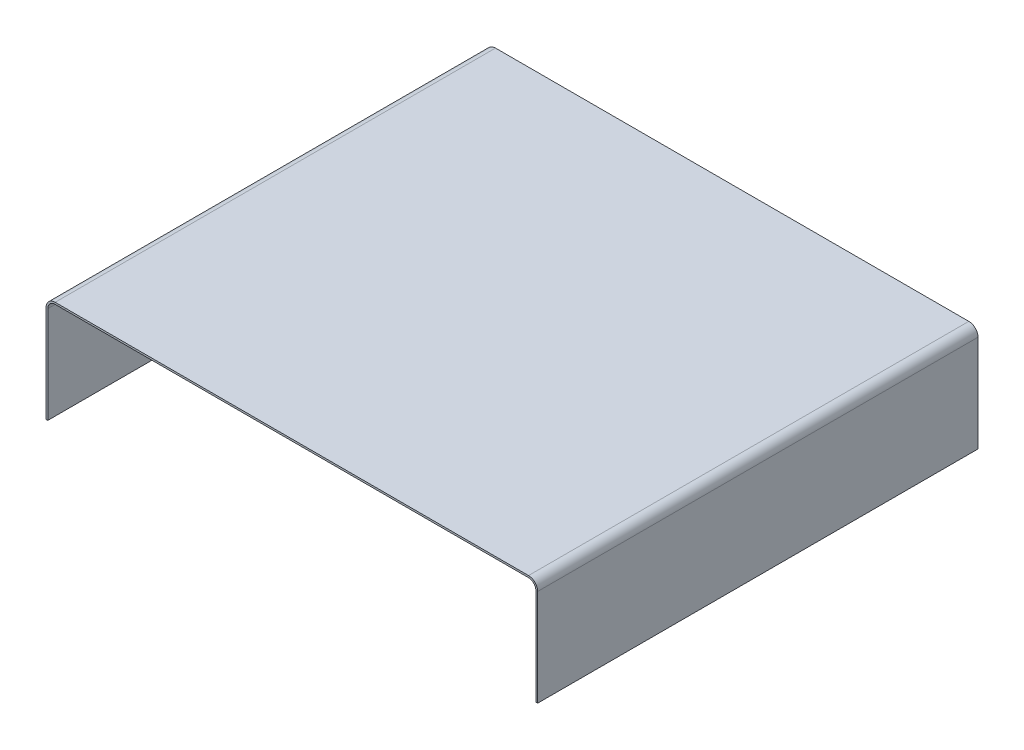
SolidWorks part; units mm, degrees
material "Plain Carbon Steel"
ref_plane "Front Plane" through (0, 0, 0) normal (0, 0, 1) x (1, 0, 0)
ref_plane "Top Plane" through (0, 0, 0) normal (0, 1, 0) x (1, 0, 0)
ref_plane "Right Plane" through (0, 0, 0) normal (1, 0, 0) x (0, 0, -1)
sketch "Sketch1" plane through (0, 0, 0) normal (0, 0, 1) x (1, 0, 0)
  line L1 (10, 0) -> (526, 0)
  line L2 (0, -10) -> (0, -115.5)
  line L4 (536, -10) -> (536, -115.5)
  arc A0 (536, -10) -> (526, 0) centre (526, -10) ccw
  arc A1 (10, 0) -> (0, -10) centre (10, -10) ccw
  point P7 (536, 0)
  point P10 (0, 0)
  dimension "D4" = 10
  dimension "D1" = 536
  dimension "D2" = 115.5
  dimension "D3" = 115.5
extrude "Extrude-Thin1" add sketch "Sketch1" along normal blind 480 thin
